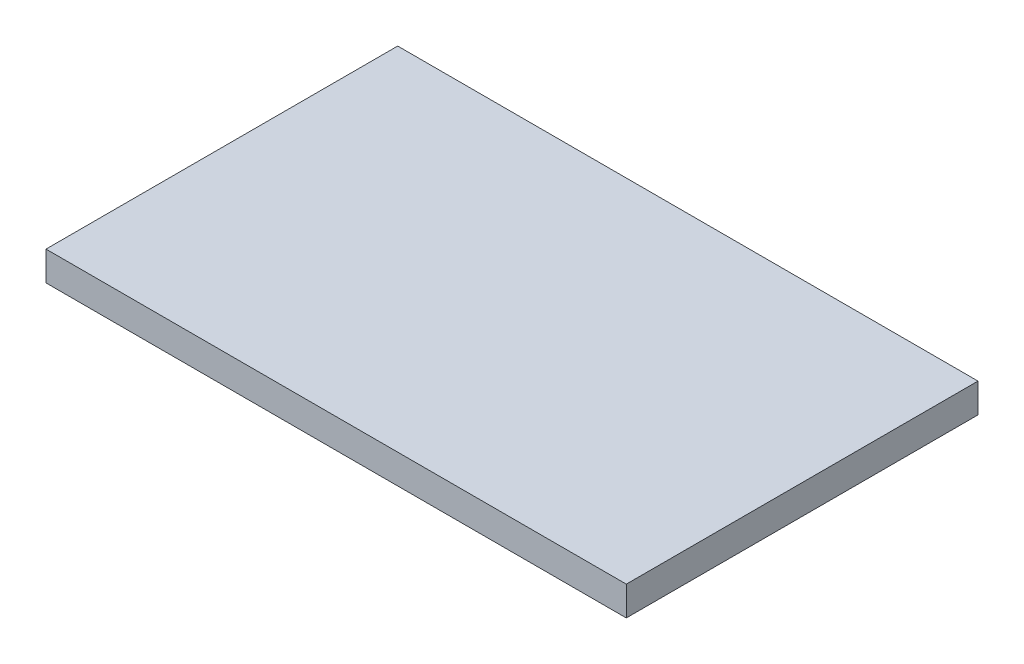
from build123d import *

# Parameters (mm, degrees)
SKETCH_1_W      = 99
SKETCH_1_H      = 5
EXTRUDE_1_DEPTH = 30


with BuildPart() as part:
    # 草图1 → 凸台-拉伸1 (new, symmetric)
    with BuildSketch(Plane.XY):
        Rectangle(SKETCH_1_W, SKETCH_1_H)
    extrude(amount=EXTRUDE_1_DEPTH, both=True)


solid = part.part
